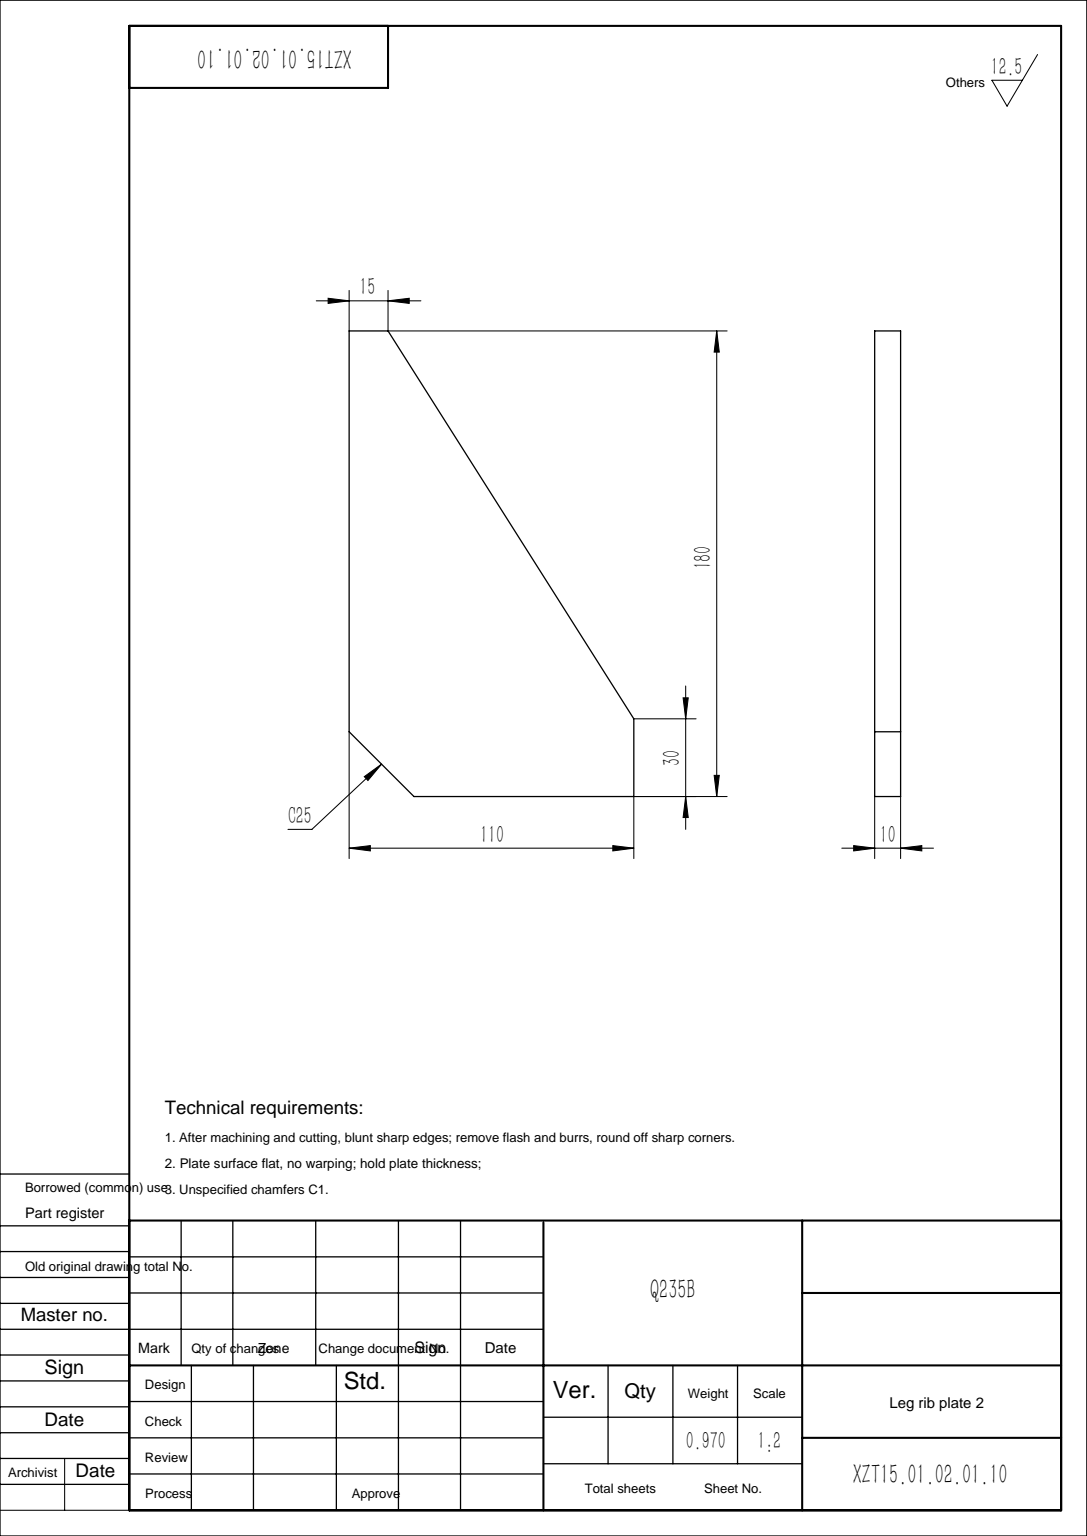
from build123d import *

# Parameters (mm, degrees)
BOSS_EXTRUDE1_DEPTH = 5
CHAMFER1_SIZE       = 25


with BuildPart() as part:
    # Sketch1 → Boss-Extrude1 (new, symmetric)
    with BuildSketch(Plane.XY):
        Polygon((0, 0), (110, 0), (110, 30), (15, 180), (0, 180), align=None)
    extrude(amount=BOSS_EXTRUDE1_DEPTH, both=True)

    # Chamfer1
    chamfer1_edges = [part.edges().sort_by_distance(p)[0] for p in [
        (0, 0, 0),
    ]]
    chamfer(chamfer1_edges, length=CHAMFER1_SIZE)


solid = part.part
